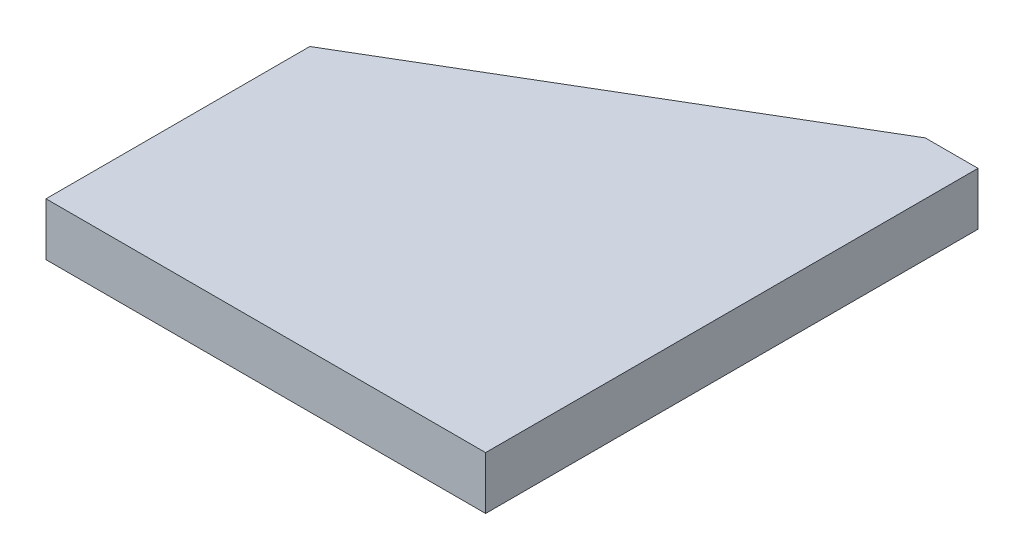
from build123d import *

# Parameters (mm, degrees)
EXTRUDE_1_DEPTH = 30


with BuildPart() as part:
    # 草图1 → 凸台-拉伸1 (new body)
    with BuildSketch(Plane(origin=(0, 0, 0), x_dir=(1, 0, 0), z_dir=(0, 1, 0))):
        Polygon((162.790697674, 182.325581395), (132.790697674, 182.325581395), (-87.209302326, 52.325581395), (-87.209302326, -97.674418605), (162.790697674, -97.674418605), align=None)
    extrude(amount=EXTRUDE_1_DEPTH)


solid = part.part
